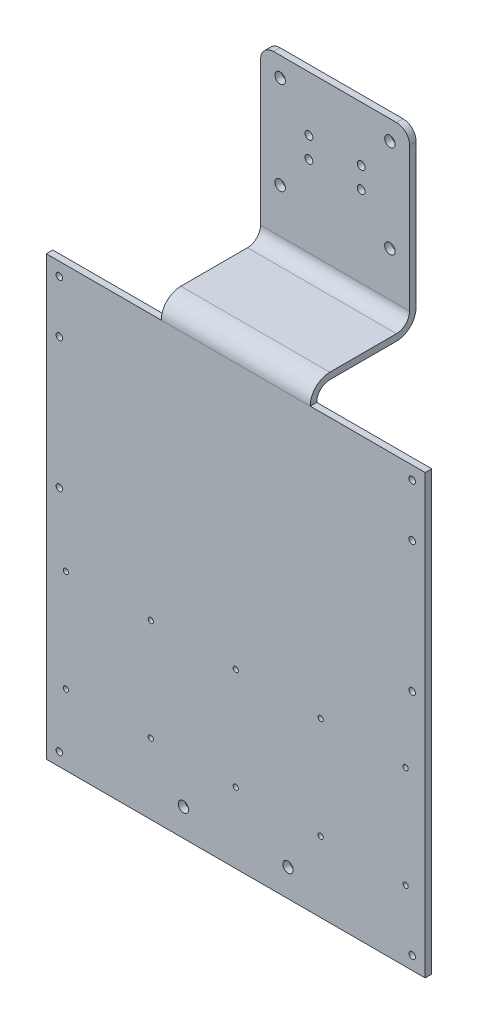
from build123d import *

# Parameters (mm, degrees)
SKETCH1_W           = 290
SKETCH1_H           = 350
BOSS_EXTRUDE1_DEPTH = 5
SKETCH2_W           = 114
SKETCH2_H           = 5
BOSS_EXTRUDE2_DEPTH = 81
SKETCH3_W           = 114
SKETCH3_H           = 5
BOSS_EXTRUDE3_DEPTH = 135
FILLET1_R           = 10
SKETCH4_W           = 88
SKETCH4_H           = 15
CUT_EXTRUDE1_DEPTH  = 120
FILLET2_R           = 15
FILLET3_R           = 10
SKETCH5_R           = 4
CUT_EXTRUDE2_DEPTH  = 120
SKETCH7_R           = 2
CUT_EXTRUDE3_DEPTH  = 10
SKETCH8_R           = 3
CUT_EXTRUDE4_DEPTH  = 10
SKETCH9_R           = 4
CUT_EXTRUDE5_DEPTH  = 10
SKETCH10_R          = 2.5
CUT_EXTRUDE6_DEPTH  = 10
SKETCH11_R          = 2.5
CUT_EXTRUDE7_DEPTH  = 10


with BuildPart() as part:
    # Sketch1 → Boss-Extrude1 (new body)
    with BuildSketch(Plane.XY):
        Rectangle(SKETCH1_W, SKETCH1_H)
    extrude(amount=BOSS_EXTRUDE1_DEPTH)

    # Sketch2 → Boss-Extrude2 (add)
    with BuildSketch(Plane.XY.offset(5)):
        with Locations((0, 172.5)):
            Rectangle(SKETCH2_W, SKETCH2_H)
    extrude(amount=-BOSS_EXTRUDE2_DEPTH)

    # Sketch3 → Boss-Extrude3 (add)
    with BuildSketch(Plane(origin=(0, 170, 0), x_dir=(-1, 0, 0), z_dir=(0, -1, 0))):
        with Locations((0, 73.5)):
            Rectangle(SKETCH3_W, SKETCH3_H)
    extrude(amount=-BOSS_EXTRUDE3_DEPTH)

    # Fillet1
    fillet1_edges = [part.edges().sort_by_distance(p)[0] for p in [
        (0, 170, 0),
        (0, 175, -71),
    ]]
    fillet(fillet1_edges, radius=FILLET1_R)

    # Sketch4 → Cut-Extrude1 (cut)
    with BuildSketch(Plane(origin=(0, 0, 0), x_dir=(-1, 0, 0), z_dir=(0, 0, -1))):
        with Locations((101, 167.5)):
            Rectangle(SKETCH4_W, SKETCH4_H)
        with Locations((-101, 167.5)):
            Rectangle(SKETCH4_W, SKETCH4_H)
    extrude(amount=-CUT_EXTRUDE1_DEPTH, mode=Mode.SUBTRACT)

    # Fillet2
    fillet2_edges = [part.edges().sort_by_distance(p)[0] for p in [
        (0, 175, 5),
        (0, 170, -76),
    ]]
    fillet(fillet2_edges, radius=FILLET2_R)

    # Fillet3
    fillet3_edges = [part.edges().sort_by_distance(p)[0] for p in [
        (57, 305, -73.5),
        (-57, 305, -73.5),
    ]]
    fillet(fillet3_edges, radius=FILLET3_R)

    # Sketch5 → Cut-Extrude2 (cut)
    with BuildSketch(Plane(origin=(0, 0, -76), x_dir=(-1, 0, 0), z_dir=(0, 0, -1))):
        with Locations((42, 290)):
            Circle(SKETCH5_R)
        with Locations((-42, 290)):
            Circle(SKETCH5_R)
        with Locations((42, 219)):
            Circle(SKETCH5_R)
        with Locations((-42, 219)):
            Circle(SKETCH5_R)
    extrude(amount=-CUT_EXTRUDE2_DEPTH, mode=Mode.SUBTRACT)

    # Sketch7 → Cut-Extrude3 (cut)
    with BuildSketch(Plane(origin=(0, 0, 0), x_dir=(-1, 0, 0), z_dir=(0, 0, -1))):
        with Locations((-130, -121)):
            Circle(SKETCH7_R)
        with Locations((-65, -121)):
            Circle(SKETCH7_R)
        with Locations((0, -121)):
            Circle(SKETCH7_R)
        with Locations((65, -121)):
            Circle(SKETCH7_R)
        with Locations((130, -121)):
            Circle(SKETCH7_R)
        with Locations((130, -43)):
            Circle(SKETCH7_R)
        with Locations((65, -43)):
            Circle(SKETCH7_R)
        with Locations((0, -43)):
            Circle(SKETCH7_R)
        with Locations((-65, -43)):
            Circle(SKETCH7_R)
        with Locations((-130, -43)):
            Circle(SKETCH7_R)
    extrude(amount=-CUT_EXTRUDE3_DEPTH, mode=Mode.SUBTRACT)

    # Sketch8 → Cut-Extrude4 (cut)
    with BuildSketch(Plane(origin=(0, 0, -76), x_dir=(-1, 0, 0), z_dir=(0, 0, -1))):
        with Locations((-20, 247)):
            Circle(SKETCH8_R)
        with Locations((-20, 263)):
            Circle(SKETCH8_R)
        with Locations((20, 263)):
            Circle(SKETCH8_R)
        with Locations((20, 247)):
            Circle(SKETCH8_R)
    extrude(amount=-CUT_EXTRUDE4_DEPTH, mode=Mode.SUBTRACT)

    # Sketch9 → Cut-Extrude5 (cut)
    with BuildSketch(Plane(origin=(0, 0, 0), x_dir=(-1, 0, 0), z_dir=(0, 0, -1))):
        with Locations((40, -154)):
            Circle(SKETCH9_R)
        with Locations((-40, -154)):
            Circle(SKETCH9_R)
    extrude(amount=-CUT_EXTRUDE5_DEPTH, mode=Mode.SUBTRACT)

    # Sketch10 → Cut-Extrude6 (cut)
    with BuildSketch(Plane(origin=(0, 0, 0), x_dir=(-1, 0, 0), z_dir=(0, 0, -1))):
        with Locations((-135, -165)):
            Circle(SKETCH10_R)
        with Locations((135, -165)):
            Circle(SKETCH10_R)
        with Locations((135, 150)):
            Circle(SKETCH10_R)
        with Locations((-135, 150)):
            Circle(SKETCH10_R)
    extrude(amount=-CUT_EXTRUDE6_DEPTH, mode=Mode.SUBTRACT)

    # Sketch11 → Cut-Extrude7 (cut)
    with BuildSketch(Plane(origin=(0, 0, 0), x_dir=(-1, 0, 0), z_dir=(0, 0, -1))):
        with Locations((135, 110)):
            Circle(SKETCH11_R)
        with Locations((135, 10)):
            Circle(SKETCH11_R)
        with Locations((-135, 110)):
            Circle(SKETCH11_R)
        with Locations((-135, 10)):
            Circle(SKETCH11_R)
    extrude(amount=-CUT_EXTRUDE7_DEPTH, mode=Mode.SUBTRACT)


solid = part.part
